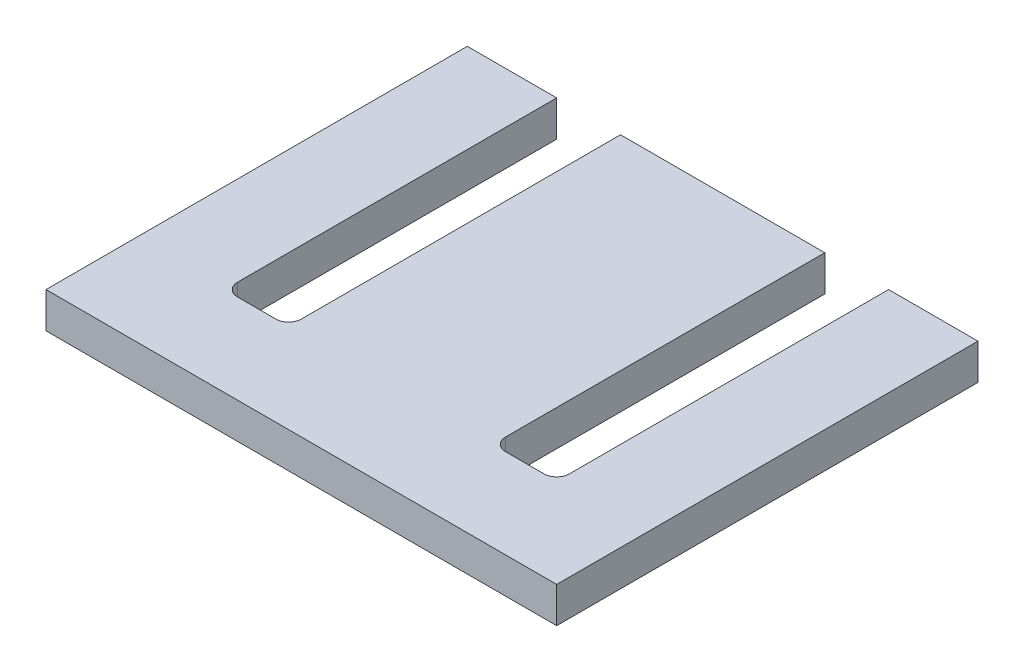
SolidWorks part; units mm, degrees
ref_plane "前视基准面" through (0, 0, 0) normal (0, 0, 1) x (1, 0, 0)
ref_plane "上视基准面" through (0, 0, 0) normal (0, 1, 0) x (1, 0, 0)
ref_plane "右视基准面" through (0, 0, 0) normal (1, 0, 0) x (0, 0, -1)
sketch "草图1" plane through (0, 0, 0) normal (0, 1, 0) x (1, 0, 0)
  line L1 (-100, -82.5) -> (100, -82.5)
  line L2 (-100, -82.5) -> (-100, 82.5)
  line L3 (-100, 82.5) -> (100, 82.5)
  line L4 (100, -82.5) -> (100, 82.5)
  line L5 (-100, -82.5) -> (100, 82.5) construction
  line L6 (-100, 82.5) -> (100, -82.5) construction
  point P0 (0, 0)
  dimension "D1" = 200
  dimension "D2" = 165
extrude "凸台-拉伸1" add sketch "草图1" along normal blind 14
sketch "草图2" plane through (0, 0, 0) normal (0, -1, 0) x (1, 0, 0)
  line L0 (65, -82.5) -> (65, 47.5)
  line L1 (100, -82.5) -> (-100, -82.5) construction
  line L2 (65, 47.5) -> (40, 47.5)
  line L3 (40, 47.5) -> (40, -82.5)
  line L4 (40, -82.5) -> (65, -82.5)
  line L5 (100, 82.5) -> (100, -82.5) construction
  line L6 (0, 0) -> (0, 82.5) construction
  line L7 (-100, 82.5) -> (100, 82.5) construction
  line L8 (-40, -82.5) -> (-65, -82.5)
  line L9 (-40, 47.5) -> (-40, -82.5)
  line L10 (-65, 47.5) -> (-40, 47.5)
  line L11 (-65, -82.5) -> (-65, 47.5)
  dimension "D1" = 25
  dimension "D2" = 130
  dimension "D3" = 35
extrude "切除-拉伸1" cut sketch "草图2" against normal up to next
fillet "圆角1" radius 5 4 edges at (65, 7, 47.5) (40, 7, 47.5) (-40, 7, 47.5) (-65, 7, 47.5)
